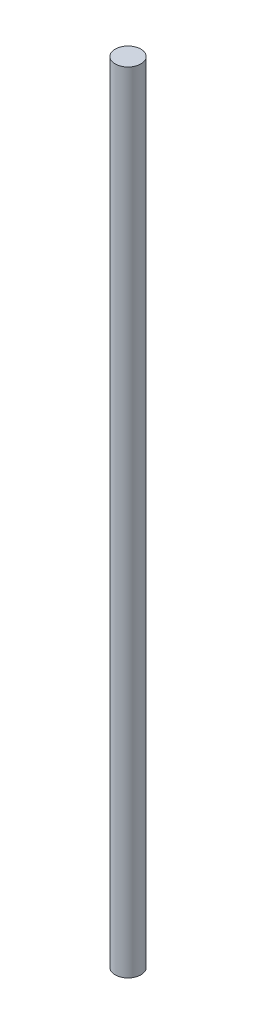
SolidWorks part; units mm, degrees
material "304"
ref_plane "Front Plane" through (0, 0, 0) normal (0, 0, 1) x (1, 0, 0)
ref_plane "Top Plane" through (0, 0, 0) normal (0, 1, 0) x (1, 0, 0)
ref_plane "Right Plane" through (0, 0, 0) normal (1, 0, 0) x (0, 0, -1)
sketch "Sketch1" plane through (0, 0, 0) normal (0, 0, 1) x (1, 0, 0)
  line L0 (0, 0) -> (0, 92)
  line L1 (0, 0) -> (1.5, 0)
  line L2 (1.5, 0) -> (1.5, 92)
  line L3 (1.5, 92) -> (0, 92)
  dimension "D1" = 92
  dimension "D2" = 1.5
revolve "Revolve1" add sketch "Sketch1" angle 360 about L0
cosmetic thread "Cosmetic Thread1" parameters "D1"=5, "D2"=2.999
